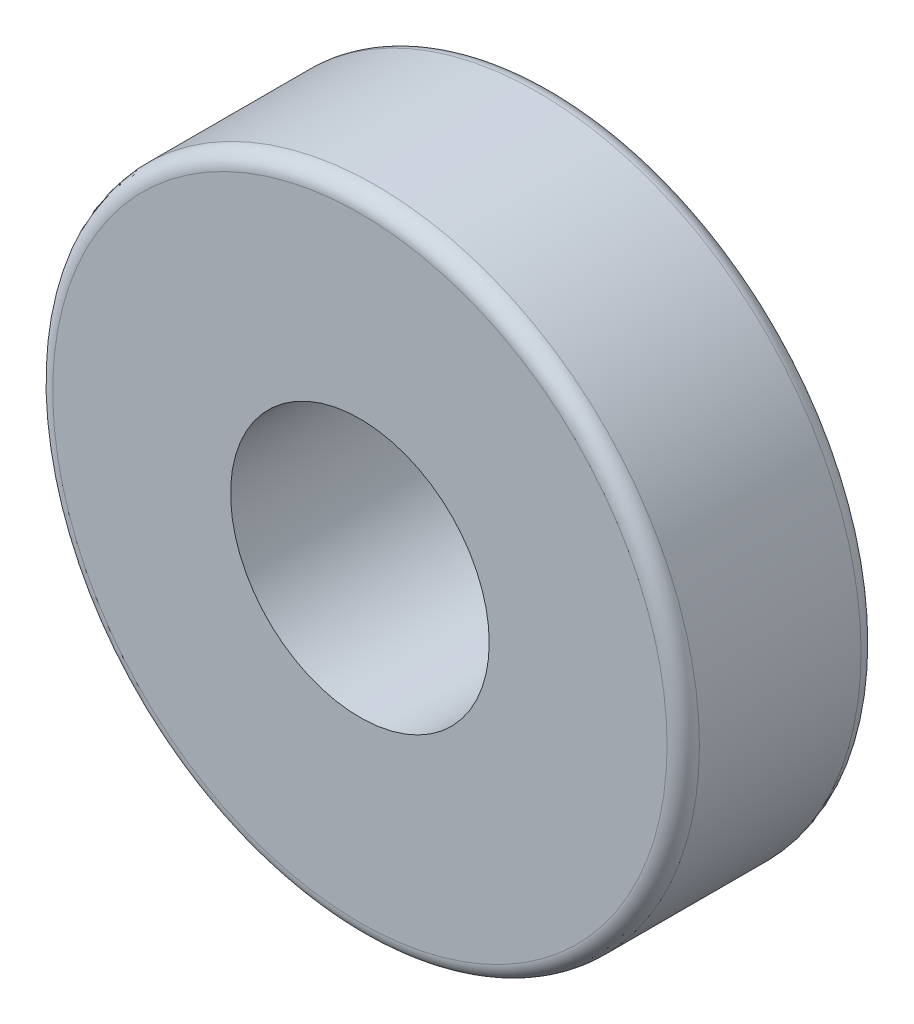
SolidWorks part; units mm, degrees
material "A3"
ref_plane "前视基准面" through (0, 0, 0) normal (0, 0, 1) x (1, 0, 0)
ref_plane "上视基准面" through (0, 0, 0) normal (0, 1, 0) x (1, 0, 0)
ref_plane "右视基准面" through (0, 0, 0) normal (1, 0, 0) x (0, 0, -1)
sketch "草图1" plane through (0, 0, 0) normal (0, 0, 1) x (1, 0, 0)
  circle A0 centre (0, 0) radius 4
  circle A1 centre (0, 0) radius 10
  dimension "D1" = 8
  dimension "D2" = 20
extrude "凸台-拉伸1" add sketch "草图1" along normal blind 6
fillet "圆角1" radius 0.5 2 edges at (10, 0, 0) (10, 0, 6)
